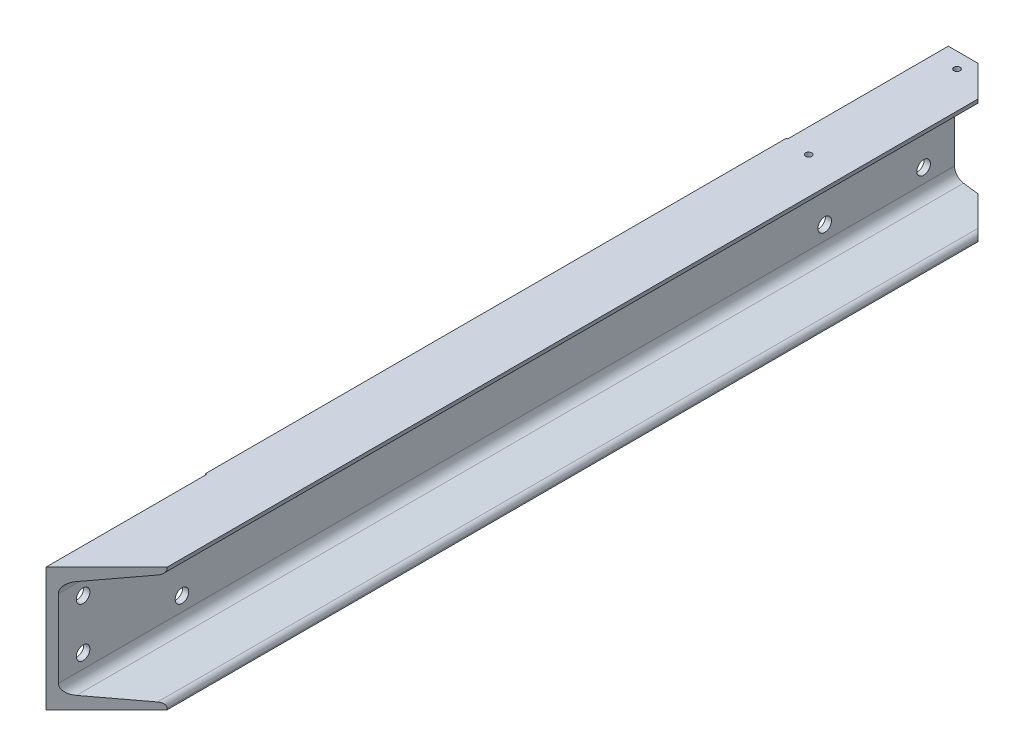
SolidWorks part; units mm, degrees
material "1023 carbon steel plate (SS)"
ref_plane "Front Plane" through (0, 0, 0) normal (0, 0, 1) x (1, 0, 0)
ref_plane "Top Plane" through (0, 0, 0) normal (0, 1, 0) x (1, 0, 0)
ref_plane "Right Plane" through (0, 0, 0) normal (1, 0, 0) x (0, 0, -1)
sketch "Sketch1" plane through (0, 0, 0) normal (0, 0, 1) x (1, 0, 0)
  line L0 (0, 0) -> (0, -100)
  line L1 (0, -100) -> (50, -100)
  line L2 (0, 0) -> (50, 0)
  line L3 (50, 0) -> (50, -1.0747)
  line L4 (50, -100) -> (50, -98.9253)
  line L5 (46.1263, -5.5309) -> (13.317, -10.1419)
  line L6 (6, -18.5592) -> (6, -81.4408)
  line L7 (13.317, -89.8581) -> (46.1263, -94.4691)
  line L8 (25, 0) -> (25, -8.5) construction
  line L9 (25, -100) -> (25, -91.5) construction
  arc A0 (6, -81.4408) -> (13.317, -89.8581) centre (14.5, -81.4408) ccw
  arc A1 (13.317, -10.1419) -> (6, -18.5592) centre (14.5, -18.5592) ccw
  arc A2 (50, -98.9253) -> (46.1263, -94.4691) centre (45.5, -98.9253) ccw
  arc A3 (50, -1.0747) -> (46.1263, -5.5309) centre (45.5, -1.0747) cw
  dimension "D8" = 8.5
  dimension "D9" = 4.5
  dimension "D1" = 100
  dimension "D2" = 50
  dimension "D3" = 50
  dimension "D4" = 6
  dimension "D5" = 8.5
  dimension "D6" = 8.5
  dimension "D7" = 98
extrude "Boss-Extrude1" add sketch "Sketch1" along normal blind 750
sketch "Sketch2" plane through (0, 0, 0) normal (0, 1, 0) x (1, 0, 0)
  line L0 (258.9926, -472.0074) -> (0, -731)
  line L2 (45.0448, -785.8728) -> (459.457, -587.6756)
  line L3 (459.457, -587.6756) -> (258.9926, -472.0074)
  line L4 (0, -750) -> (0, 0) construction
  line L5 (0, -731) -> (-59.7772, -772.2622)
  line L6 (-59.7772, -772.2622) -> (30.8414, -818.1599)
  line L7 (30.8414, -818.1599) -> (45.0448, -785.8728)
  line L8 (25, 0) -> (50, -25)
  line L9 (50, 0) -> (0, 0) construction
  line L10 (50, -750) -> (50, 0) construction
  line L11 (50, -25) -> (50, 48.4172)
  line L12 (50, 48.4172) -> (25, 0)
  dimension "D1" = 45
  dimension "D2" = 731
  dimension "D3" = 25
  dimension "D4" = 25
extrude "Cut-Extrude1" cut sketch "Sketch2" against normal blind 730
sketch "Sketch3" plane through (0, 0, 0) normal (-1, 0, 0) x (0, 0, 1)
  line L0 (130, 38.7018) -> (130, -162.7252)
  line L1 (130, -162.7252) -> (-125.6336, -119.6063)
  line L2 (-125.6336, -119.6063) -> (-100.4183, 29.8844)
  line L3 (-100.4183, 29.8844) -> (130, 38.7018)
  line L4 (0, 0) -> (0, -100) construction
  line L5 (731, -100) -> (731, 0) construction
  line L6 (846.7925, 272.7759) -> (600, 272.7759)
  line L7 (846.7925, 272.7759) -> (846.7925, -138.7018)
  line L8 (846.7925, -138.7018) -> (600, -138.7018)
  line L9 (600, 272.7759) -> (600, -138.7018)
  line L10 (846.7925, 272.7759) -> (600, -138.7018) construction
  line L11 (846.7925, -138.7018) -> (600, 272.7759) construction
  point P6 (723.3962, 67.0371)
  dimension "D1" = 130
  dimension "D2" = 131
extrude "Cut-Extrude2" cut sketch "Sketch3" against normal blind 1
sketch "Sketch4" plane through (1, 0, 0) normal (-1, 0, 0) x (0, 0, 1)
  line L0 (0, 0) -> (0, -100) construction
  line L2 (730, 0) -> (730, -100) construction
  circle A0 centre (25, -30) radius 5.5
  circle A1 centre (105, -30) radius 5.5
  circle A2 centre (25, -70) radius 5.5
  circle A3 centre (105, -70) radius 5.5
  circle A4 centre (625, -30) radius 5.5
  circle A5 centre (705, -70) radius 5.5
  circle A6 centre (625, -70) radius 5.5
  circle A7 centre (705, -30) radius 5.5
  point P14 (0, -50)
  dimension "D5" = 11
  dimension "D1" = 40
  dimension "D2" = 80
  dimension "D3" = 20
  dimension "D4" = 25
  dimension "D6" = 25
  dimension "D7" = 80
extrude "Cut-Extrude3" cut sketch "Sketch4" against normal blind 10
sketch "Sketch10" plane through (0, 0, 0) normal (0, 1, 0) x (1, 0, 0)
  line L0 (25, 0) -> (1, 0) construction
  line L1 (0, -600) -> (0, -130) construction
  circle A0 centre (20.5, -12.5) radius 2
  circle A1 centre (20.5, -132.5) radius 2
  dimension "D3" = 4
  dimension "D1" = 120
  dimension "D2" = 12.5
  dimension "D4" = 20.5
hole_wizard "M6 Tapped Hole3" positions "Sketch11" profile "Sketch12" tap size "M6" standard "ISO"
sketch "Sketch11" plane through (0, 0, 0) normal (0, 1, 0) x (1, 0, 0)
  point P0 (20.5, -12.5)
  point P3 (20.5, -132.5)
sketch "Sketch12" plane through (20.5, 0, 12.5) normal (1, 0, 0) x (0, 0, 1)
  line L0 (0, 0) -> (0, 16.5022)
  line L1 (0, 16.5022) -> (2.5, 15)
  line L2 (2.5, 15) -> (2.5, 0)
  line L5 (2.5, 0) -> (0, 0)
  line L10 (0, 16.5022) -> (-2.5, 15) construction
  line L11 (0, -6.35) -> (0, 107.95) construction
  dimension "螺纹孔钻头直径" = 5
  dimension "螺纹孔钻头深度" = 15
  dimension "导头角度" = 118
cosmetic thread "Cosmetic thread 3" parameters "D1"=12, "D2"=6
cosmetic thread "Cosmetic thread 4" parameters "D1"=12, "D2"=6
